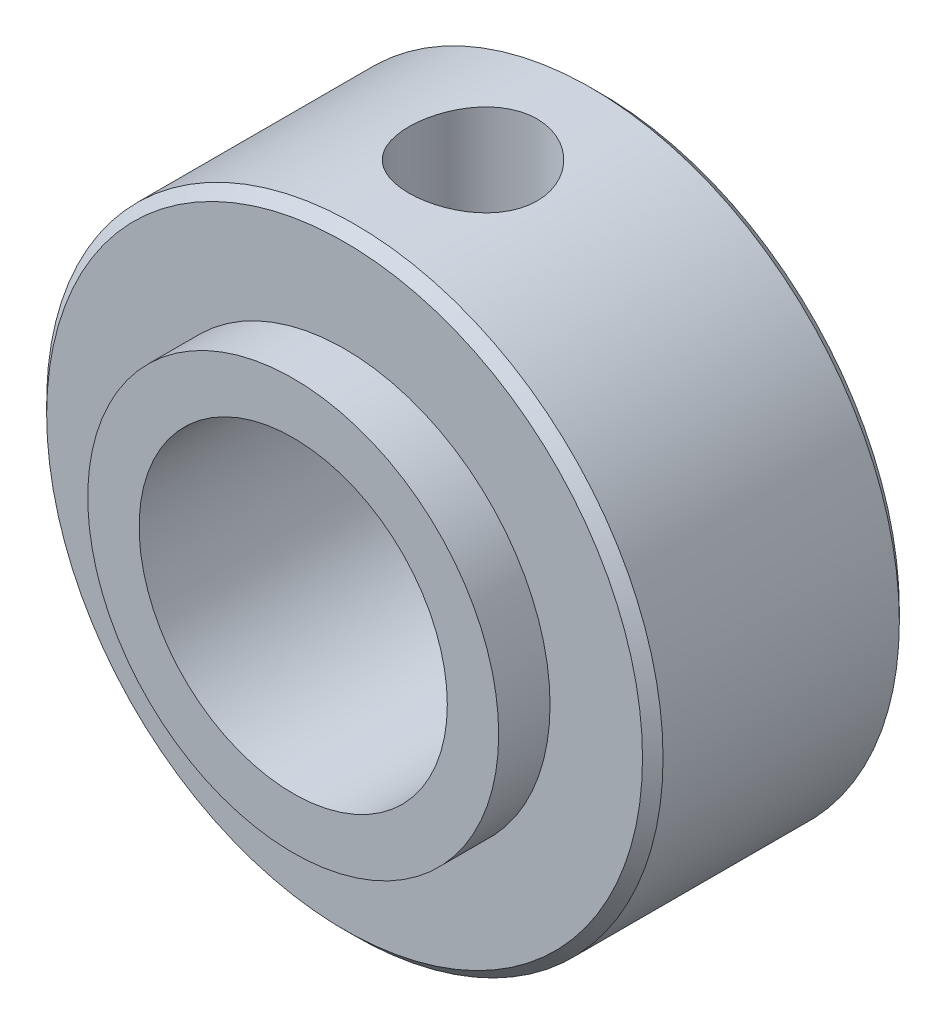
from build123d import *

# Parameters (mm, degrees)
SKETCH1_R           = 6
BOSS_EXTRUDE1_DEPTH = 5
SKETCH2_R           = 4
BOSS_EXTRUDE2_DEPTH = 1
SKETCH3_R           = 3
CUT_EXTRUDE1_DEPTH  = 11.392304845
CHAMFER1_SIZE       = 0.2


with BuildPart() as part:
    # Sketch1 → Boss-Extrude1 (new body)
    with BuildSketch(Plane.XY):
        Circle(SKETCH1_R)
    extrude(amount=BOSS_EXTRUDE1_DEPTH)

    # Sketch2 → Boss-Extrude2 (add)
    with BuildSketch(Plane.XY.offset(5)):
        Circle(SKETCH2_R)
    extrude(amount=BOSS_EXTRUDE2_DEPTH)

    # Sketch3 → Cut-Extrude1 (cut, through all)
    with BuildSketch(Plane.XY.offset(6)):
        Circle(SKETCH3_R)
    extrude(amount=-CUT_EXTRUDE1_DEPTH, mode=Mode.SUBTRACT)

    # Chamfer1
    chamfer1_edges = [part.edges().sort_by_distance(p)[0] for p in [
        (-6, 0, 0),
        (-6, 0, 5),
    ]]
    chamfer(chamfer1_edges, length=CHAMFER1_SIZE)

    # Sketch4 → M3 Tapped Hole1 (revolve, cut)
    with BuildSketch(Plane(origin=(0, 0, 2.5), x_dir=(0, 0, -1), z_dir=(1, 0, 0))):
        Polygon((0, 0), (0, 8.251075774), (1.25, 7.5), (1.25, 0), align=None)
    revolve(axis=Axis((0, -6.35, 2.5), (0, 1, 0)), mode=Mode.SUBTRACT)


solid = part.part
